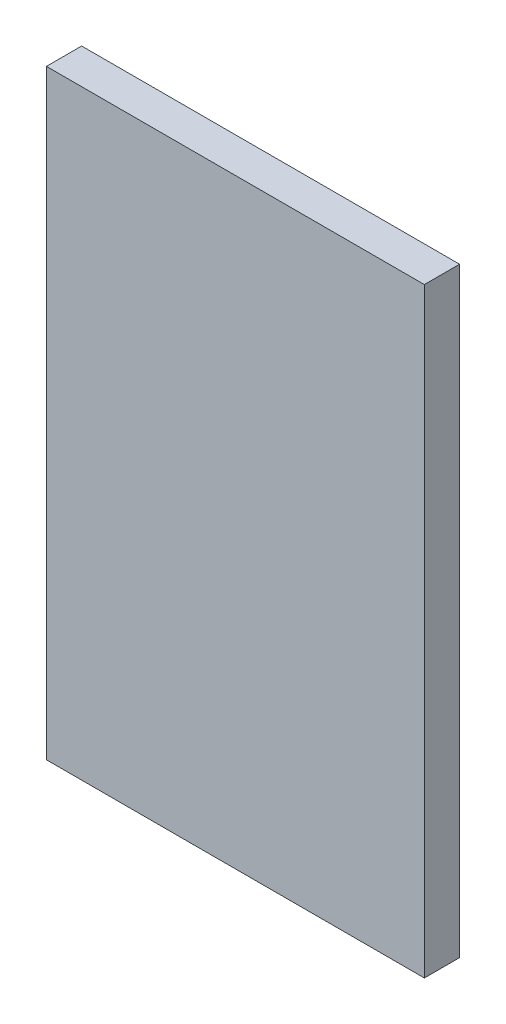
SolidWorks part; units mm, degrees
material "Q235B"
ref_plane "Front Plane" through (0, 0, 0) normal (0, 0, 1) x (1, 0, 0)
ref_plane "Top Plane" through (0, 0, 0) normal (0, 1, 0) x (1, 0, 0)
ref_plane "Right Plane" through (0, 0, 0) normal (1, 0, 0) x (0, 0, -1)
sketch "Sketch1" plane through (0, 0, 0) normal (0, 0, 1) x (1, 0, 0)
  line L1 (59, -93.75) -> (-59, -93.75)
  line L2 (59, -93.75) -> (59, 93.75)
  line L3 (59, 93.75) -> (-59, 93.75)
  line L4 (-59, -93.75) -> (-59, 93.75)
  line L5 (59, -93.75) -> (-59, 93.75) construction
  line L6 (59, 93.75) -> (-59, -93.75) construction
  point P0 (0, 0)
  dimension "D1" = 187.5
  dimension "D2" = 118
extrude "Boss-Extrude1" add sketch "Sketch1" along normal mid plane 11
